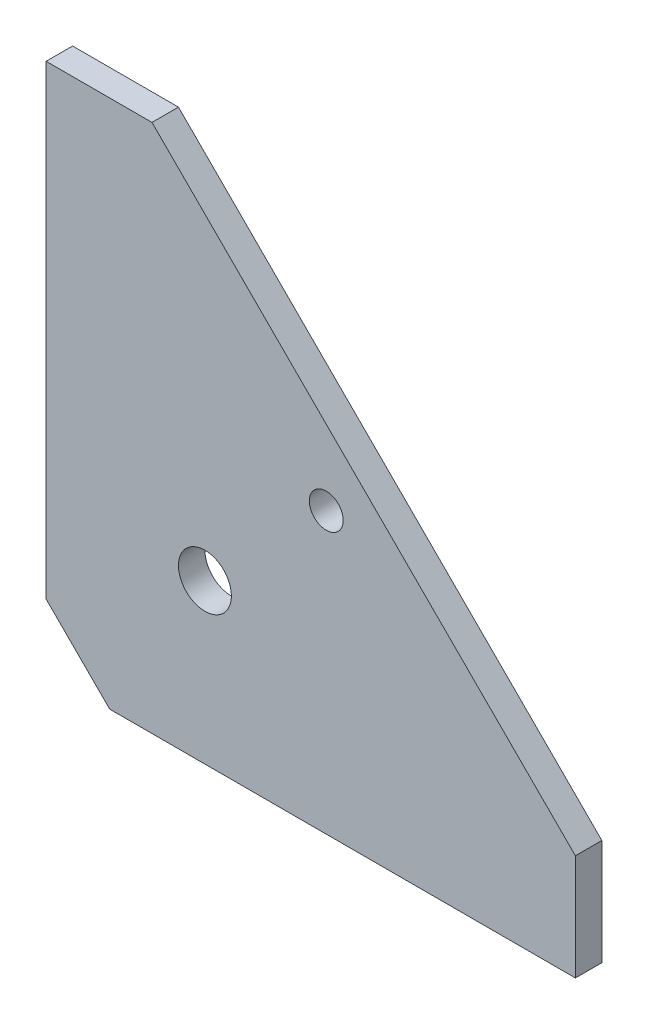
SolidWorks part; units mm, degrees
ref_plane "Front Plane" through (0, 0, 0) normal (0, 0, 1) x (1, 0, 0)
ref_plane "Top Plane" through (0, 0, 0) normal (0, 1, 0) x (1, 0, 0)
ref_plane "Right Plane" through (0, 0, 0) normal (1, 0, 0) x (0, 0, -1)
other "Configuration Table"
sketch "Sketch1" plane through (0, 0, 0) normal (0, 0, 1) x (1, 0, 0)
  line L0 (0, 0) -> (0, 500)
  line L1 (0, 0) -> (500, 0)
  line L2 (0, 500) -> (100, 500)
  line L3 (500, 0) -> (500, 100)
  line L4 (100, 500) -> (500, 100)
  dimension "D1" = 500
  dimension "D2" = 500
  dimension "D3" = 100
  dimension "D4" = 100
extrude "Boss-Extrude1" add sketch "Sketch1" along normal blind 25
sketch "Sketch2" plane through (0, 0, 25) normal (0, 0, 1) x (1, 0, 0)
  line L0 (0, 0) -> (500, 0) construction
  line L1 (0, 500) -> (0, 0) construction
  circle A0 centre (150, 150) radius 25
  dimension "D1" = 50
  dimension "D2" = 150
  dimension "D3" = 150
extrude "Cut-Extrude1" cut sketch "Sketch2" against normal blind 25
chamfer "Chamfer1" distance 60 angle 45 1 edges at (0, 0, 12.5)
sketch "Sketch3" plane through (0, 0, 25) normal (0, 0, 1) x (1, 0, 0)
  line L0 (300, 300) -> (33.5236, 33.5236) construction
  line L1 (500, 100) -> (100, 500) construction
  circle A0 centre (264.6447, 264.6447) radius 16
  dimension "D1" = 32
  dimension "D2" = 50
extrude "Cut-Extrude2" cut sketch "Sketch3" against normal through all
